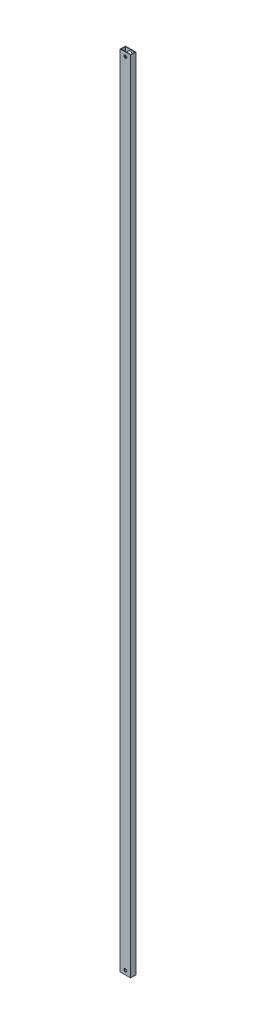
SolidWorks part; units mm, degrees
ref_plane "前视基准面" through (0, 0, 0) normal (0, 0, 1) x (1, 0, 0)
ref_plane "上视基准面" through (0, 0, 0) normal (0, 1, 0) x (1, 0, 0)
ref_plane "右视基准面" through (0, 0, 0) normal (1, 0, 0) x (0, 0, -1)
sketch "草图2" plane through (0, 0, 0) normal (0, 1, 0) x (1, 0, 0)
  line L0 (-9, 4) -> (-9, -4)
  line L1 (-10, 5) -> (10, 5)
  line L2 (-10, 5) -> (-10, -5)
  line L3 (-10, -5) -> (10, -5)
  line L4 (10, 5) -> (10, -5)
  line L5 (-10, 5) -> (10, -5) construction
  line L6 (-10, -5) -> (10, 5) construction
  line L11 (14.8467, -7.4234) -> (102.4781, -51.2391) construction
  line L12 (-41.3703, -26.2348) -> (41.3703, 26.2348) construction
  line L13 (-9, -4) -> (9, -4)
  line L14 (9, 4) -> (9, -4)
  line L15 (-9, 4) -> (9, 4)
  point P0 (0, 0)
  point P6 (0, 0)
  dimension "D2" = 10
  dimension "D3" = 20
  dimension "D1" = 1
extrude "凸台-拉伸1" add sketch "草图2" along normal blind 1546.3
hole_wizard "打孔尺寸(%根据)内六角圆柱头螺钉的类型1" positions "草图3" profile "草图4" counterbore size "M5" standard "GB" end condition through all
sketch "草图3" plane through (0, 0, -5) normal (0, 0, -1) x (-1, 0, 0)
  line L0 (-10, 773.15) -> (192.5495, 773.15) construction
  line L1 (-10, 1546.3) -> (-10, 0) construction
  line L3 (0, 1546.3) -> (0, 1461.4836) construction
  line L4 (-10, 1546.3) -> (10, 1546.3) construction
  point P0 (0, 1538.3)
  point P2 (0, 8)
  dimension "D1" = 8
sketch "草图4" plane through (0, 1538.3, -5) normal (1, 0, 0) x (0, 1, 0)
  line L0 (0, 0) -> (0, 10)
  line L1 (0, 10) -> (2.75, 10)
  line L3 (2.75, 10) -> (2.75, 5.7)
  line L4 (2.75, 5.7) -> (5, 5.7)
  line L5 (5, 5.7) -> (5, 0)
  line L7 (5, 0) -> (0, 0)
  line L11 (0, -6.35) -> (0, 107.95) construction
  dimension "通孔孔直径" = 5.5
  dimension "通孔孔深度" = 10
  dimension "柱形沉头孔直径" = 10
  dimension "柱形沉头孔深度" = 5.7
